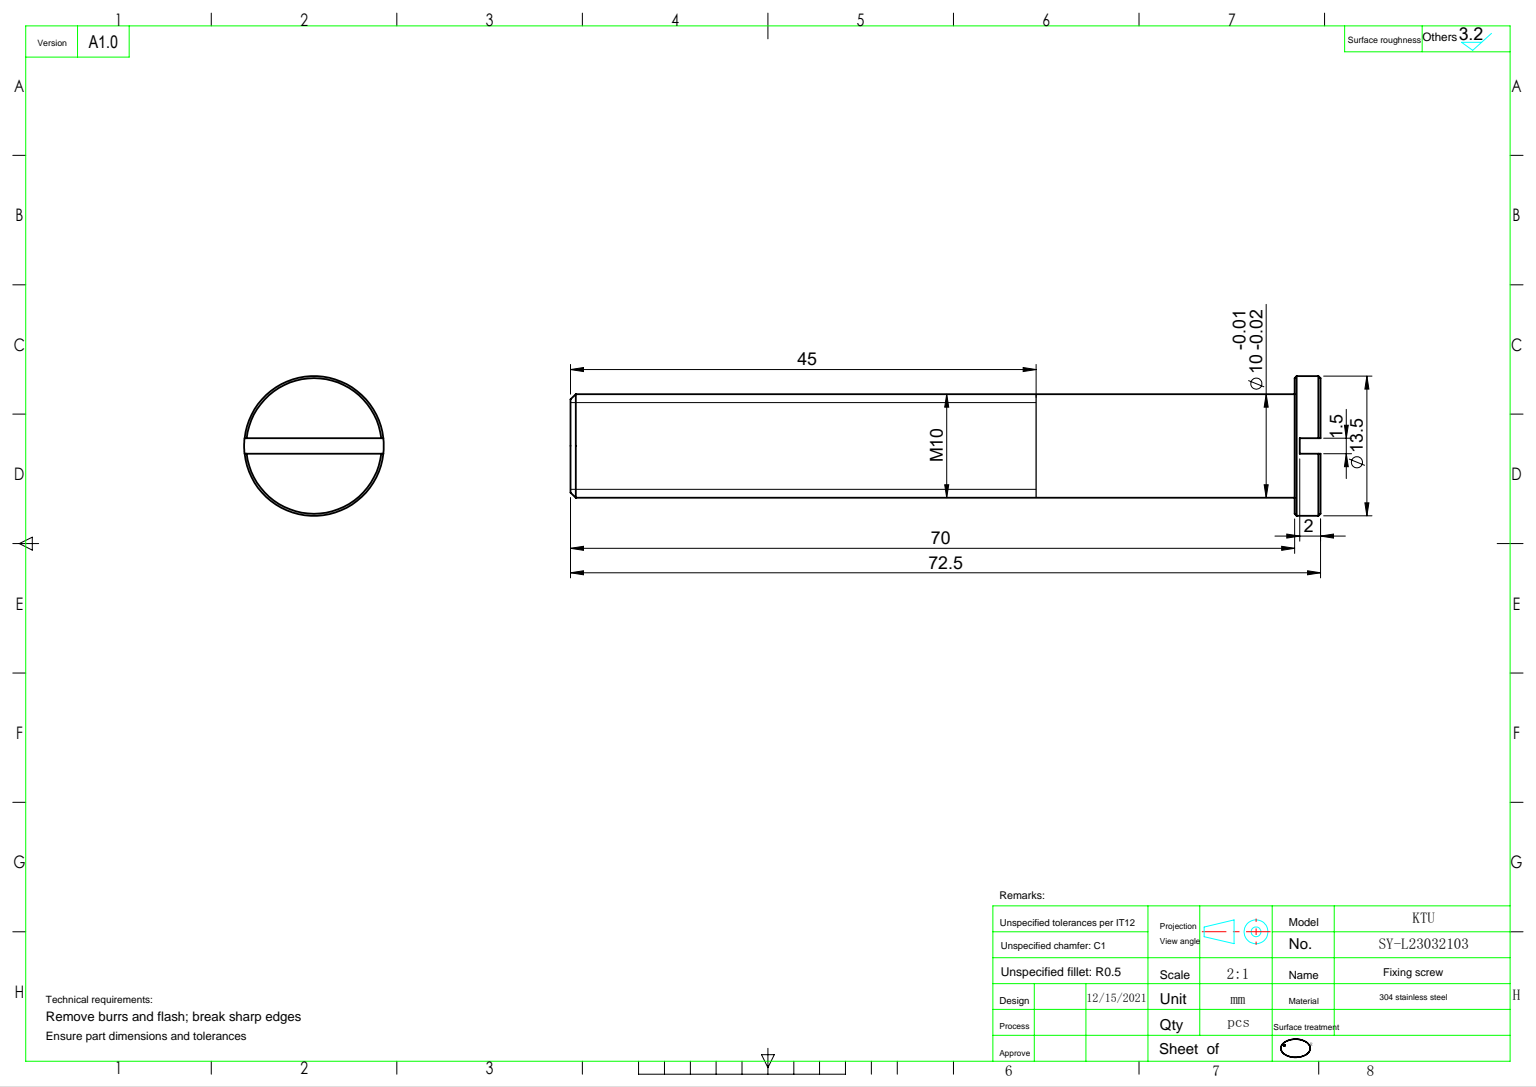
from build123d import *

# Parameters (mm, degrees)
SKETCH_4_R          = 5
EXTRUDE_3_DEPTH     = 70
SKETCH_5_R          = 6.75
EXTRUDE_4_DEPTH     = 2.5
CHAMFER_1_SIZE      = 0.5
CHAMFER_2_SIZE      = 0.2
SKETCH_6_W          = 15
SKETCH_6_H          = 1.5
CUT_EXTRUDE_1_DEPTH = 2


with BuildPart() as part:
    # 草图4 → 凸台-拉伸3 (new body)
    with BuildSketch(Plane.XY):
        Circle(SKETCH_4_R)
    extrude(amount=EXTRUDE_3_DEPTH)

    # 草图5 → 凸台-拉伸4 (add)
    with BuildSketch(Plane(origin=(0, 0, 0), x_dir=(-1, 0, 0), z_dir=(0, 0, -1))):
        Circle(SKETCH_5_R)
    extrude(amount=EXTRUDE_4_DEPTH)

    # 倒角1
    chamfer_1_edges = [part.edges().sort_by_distance(p)[0] for p in [
        (-5, 0, 70),
    ]]
    chamfer(chamfer_1_edges, length=CHAMFER_1_SIZE)

    # 倒角2
    chamfer_2_edges = [part.edges().sort_by_distance(p)[0] for p in [
        (6.75, 0, 0),
        (6.75, 0, -2.5),
    ]]
    chamfer(chamfer_2_edges, length=CHAMFER_2_SIZE)

    # 草图6 → 切除-拉伸1 (cut)
    with BuildSketch(Plane(origin=(0, 0, -2.5), x_dir=(-1, 0, 0), z_dir=(0, 0, -1))):
        Rectangle(SKETCH_6_W, SKETCH_6_H)
    extrude(amount=-CUT_EXTRUDE_1_DEPTH, mode=Mode.SUBTRACT)


solid = part.part
